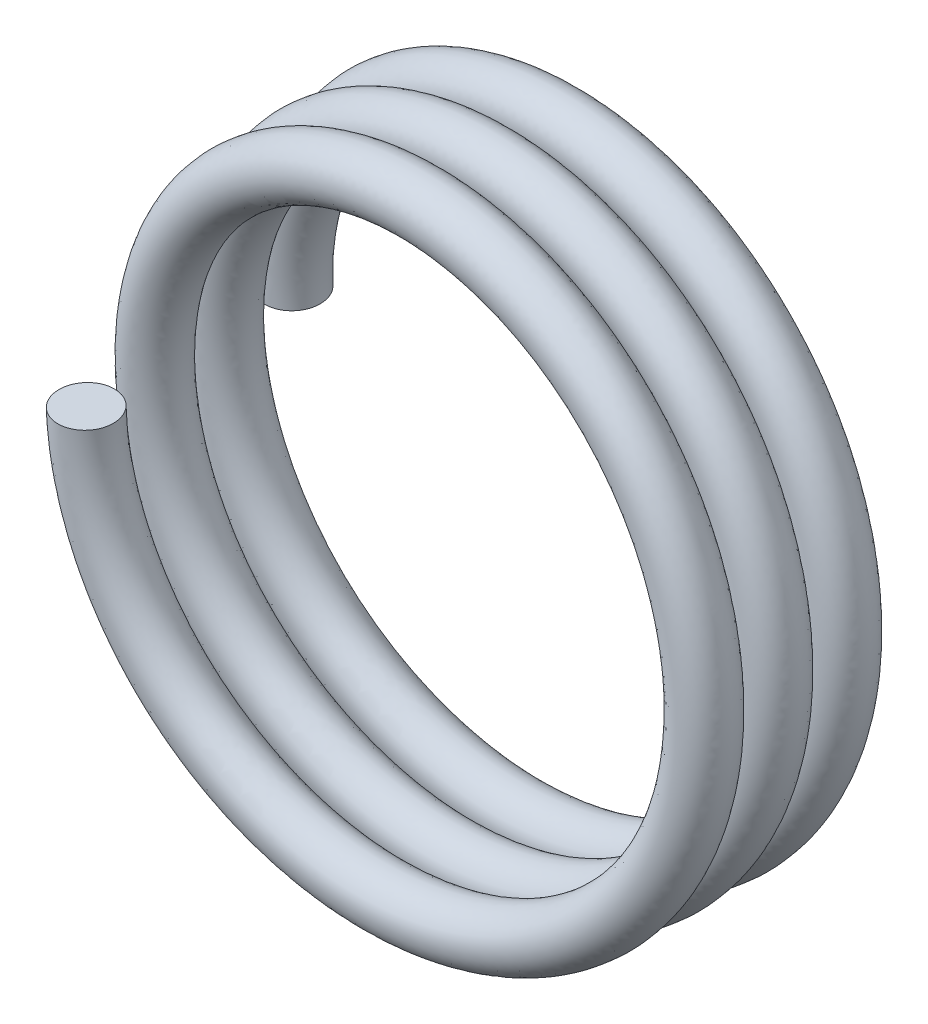
from build123d import *

# Parameters (mm, degrees)
SWEEP1_PITCH       = 1.833333333
SWEEP1_HEIGHT      = 5.5
SWEEP1_RADIUS      = 7.75
SWEEP1_START_ANGLE = -180
SWEEP1_PROFILE_R   = 0.75


with BuildPart() as part:
    # Sweep1: sweep along a helix
    with BuildLine() as sweep1_path:
        add(Helix(SWEEP1_PITCH, SWEEP1_HEIGHT, SWEEP1_RADIUS, center=(0, 0, 0), direction=(0, 0, 1), lefthand=True, mode=Mode.PRIVATE).rotate(Axis((0, 0, 0), (0, 0, 1)), SWEEP1_START_ANGLE))
    # Sweep1 profile (on start of the path) → Sweep1 (sweep)
    with BuildSketch(Plane(origin=(-7.75, 0, 0), x_dir=(0, -0.03762290084709483, 0.9992920080396169), z_dir=(-1.5637846105898416e-13, 0.9992920080396169, 0.03762290084709483))):
        Circle(SWEEP1_PROFILE_R)
    sweep(path=sweep1_path.line, is_frenet=True)


solid = part.part
